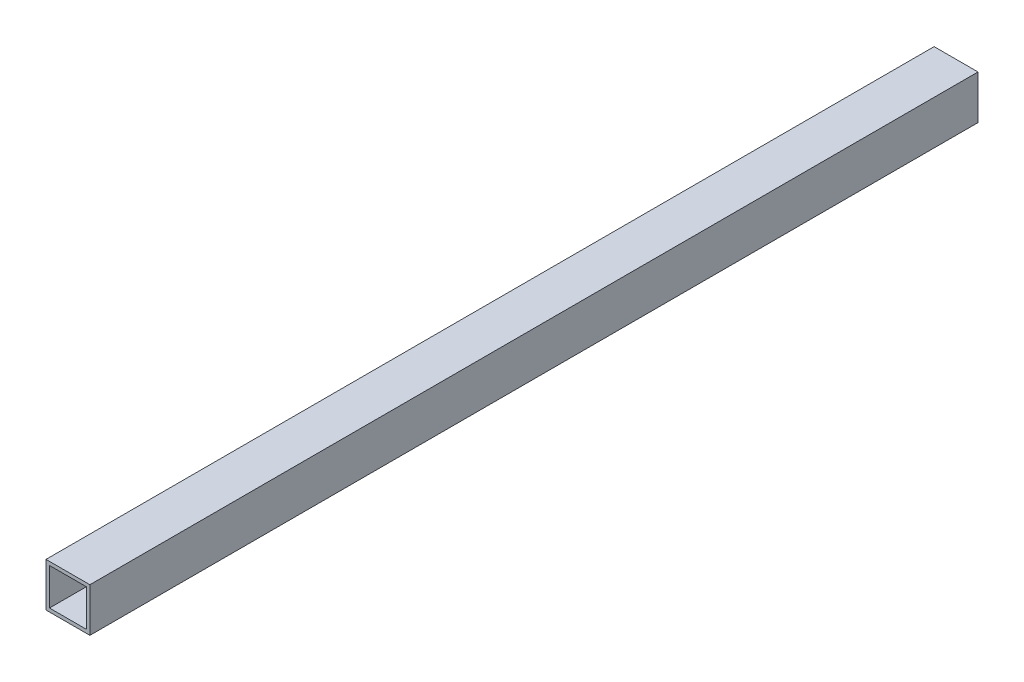
SolidWorks part; units mm, degrees
ref_plane "前视基准面" through (0, 0, 0) normal (0, 0, 1) x (1, 0, 0)
ref_plane "上视基准面" through (0, 0, 0) normal (0, 1, 0) x (1, 0, 0)
ref_plane "右视基准面" through (0, 0, 0) normal (1, 0, 0) x (0, 0, -1)
other "Configuration Table"
sketch "草图1" plane through (0, 0, 0) normal (0, 0, 1) x (1, 0, 0)
  line L0 (-25, -25) -> (25, -25)
  line L1 (25, -25) -> (25, 25)
  line L2 (25, 25) -> (-25, 25)
  line L3 (-25, 25) -> (-25, -25)
  line L4 (-21, -21) -> (21, -21)
  line L5 (21, -21) -> (21, 21)
  line L6 (21, 21) -> (-21, 21)
  line L7 (-21, 21) -> (-21, -21)
  point P0 (0, 0)
  dimension "D1" = 4
  dimension "D2" = 25
  dimension "D3" = 46
  dimension "D4" = 50
  dimension "D5" = 4
  dimension "D6" = 25
  dimension "D7" = 46
  dimension "D8" = 50
extrude "凸台-拉伸1" add sketch "草图1" against normal mid plane 1012
